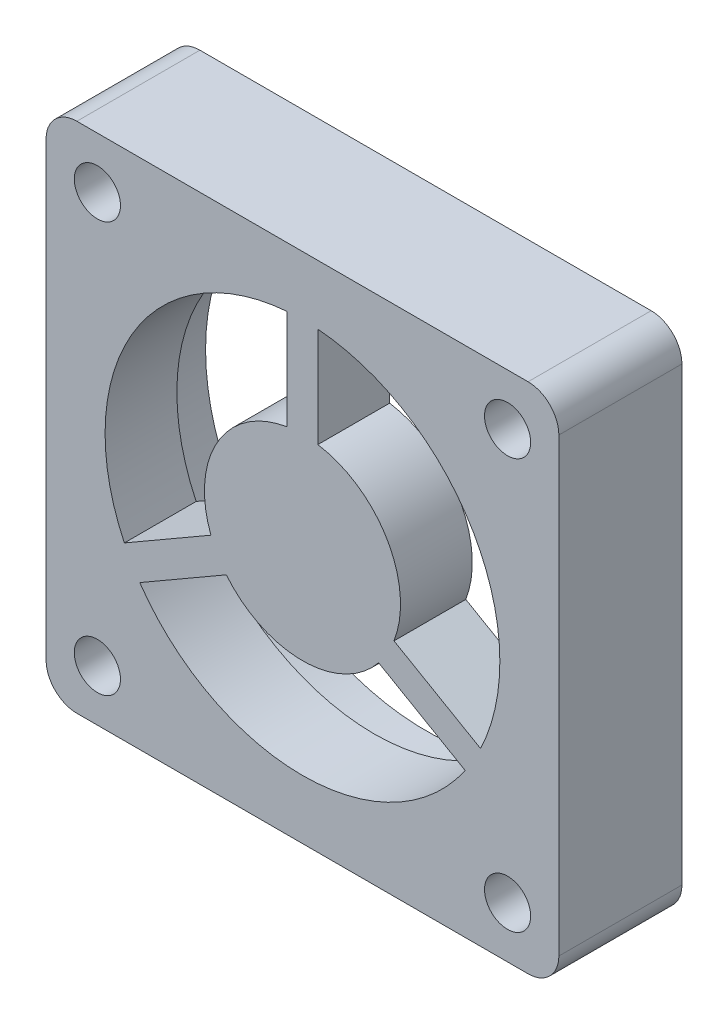
from build123d import *

# Parameters (mm, degrees)
SKETCH1_R           = 2.25
BOSS_EXTRUDE1_DEPTH = 12
CUT_EXTRUDE1_DEPTH  = 12
SKETCH3_R           = 21.449558408
CUT_EXTRUDE2_DEPTH  = 5


with BuildPart() as part:
    # Sketch1 → Boss-Extrude1 (new body)
    with BuildSketch(Plane.XY):
        with BuildLine():
            Line((-22, 25), (22, 25))
            ThreePointArc((22, 25), (24.121320344, 24.121320344), (25, 22))
            Line((25, 22), (25, -22))
            ThreePointArc((25, -22), (24.121320344, -24.121320344), (22, -25))
            Line((22, -25), (-22, -25))
            ThreePointArc((-22, -25), (-24.121320344, -24.121320344), (-25, -22))
            Line((-25, -22), (-25, 22))
            ThreePointArc((-25, 22), (-24.121320344, 24.121320344), (-22, 25))
        make_face()
        with Locations((-20, 20)):
            Circle(SKETCH1_R, mode=Mode.SUBTRACT)
        with Locations((20, 20)):
            Circle(SKETCH1_R, mode=Mode.SUBTRACT)
        with Locations((20, -20)):
            Circle(SKETCH1_R, mode=Mode.SUBTRACT)
        with Locations((-20, -20)):
            Circle(SKETCH1_R, mode=Mode.SUBTRACT)
    extrude(amount=BOSS_EXTRUDE1_DEPTH)

    # Sketch2 → Cut-Extrude1 (cut)
    with BuildSketch(Plane.XY.offset(12)):
        with BuildLine():
            Line((-1.5, 19.188784117), (-1.5, 9.440713214))
            ThreePointArc((-1.5, 9.440713214), (-8.278453932, 4.779567606), (-8.925897474, -3.421318502))
            Line((-8.925897474, -3.421318502), (-17.367974513, -8.295353953))
            ThreePointArc((-17.367974513, -8.295353953), (-16.668670521, 9.623661412), (-1.5, 19.188784117))
        make_face()
        with BuildLine():
            Line((1.5, 19.188784117), (1.5, 9.440713214))
            ThreePointArc((1.5, 9.440713214), (8.278453932, 4.779567606), (8.925897474, -3.421318502))
            Line((8.925897474, -3.421318502), (17.367974513, -8.295353953))
            ThreePointArc((17.367974513, -8.295353953), (16.668670521, 9.623661412), (1.5, 19.188784117))
        make_face()
        with BuildLine():
            Line((15.867974513, -10.893430164), (7.425897474, -6.019394713))
            ThreePointArc((7.425897474, -6.019394713), (0, -9.559135212), (-7.425897474, -6.019394713))
            Line((-7.425897474, -6.019394713), (-15.867974513, -10.893430164))
            ThreePointArc((-15.867974513, -10.893430164), (0, -19.247322824), (15.867974513, -10.893430164))
        make_face()
    extrude(amount=-CUT_EXTRUDE1_DEPTH, mode=Mode.SUBTRACT)

    # Sketch3 → Cut-Extrude2 (cut)
    with BuildSketch(Plane(origin=(0, 0, 0), x_dir=(-1, 0, 0), z_dir=(0, 0, -1))):
        Circle(SKETCH3_R)
    extrude(amount=-CUT_EXTRUDE2_DEPTH, mode=Mode.SUBTRACT)


solid = part.part
